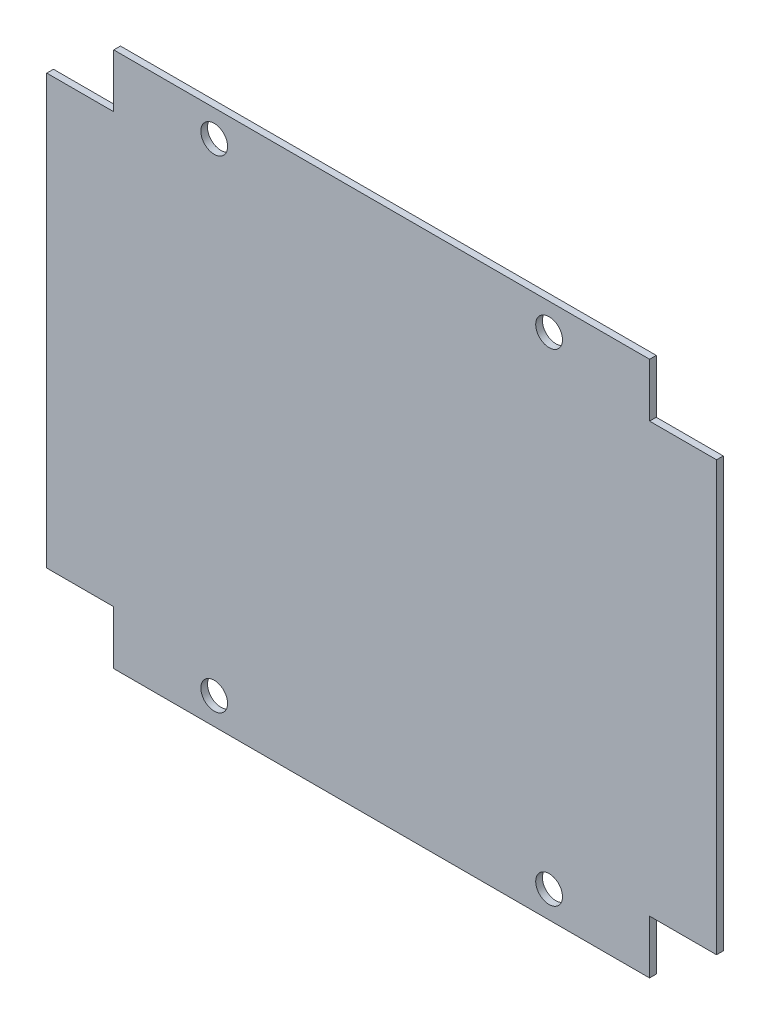
SolidWorks part; units mm, degrees
ref_plane "Front Plane" through (0, 0, 0) normal (0, 0, 1) x (1, 0, 0)
ref_plane "Top Plane" through (0, 0, 0) normal (0, 1, 0) x (1, 0, 0)
ref_plane "Right Plane" through (0, 0, 0) normal (1, 0, 0) x (0, 0, -1)
sketch "Sketch1" plane through (0, 0, 0) normal (0, 0, 1) x (1, 0, 0)
  line L0 (-40, 36) -> (40, 36) construction
  line L1 (-40, 40) -> (40, 40)
  line L2 (-50, 32) -> (-50, -32)
  line L3 (-40, -40) -> (40, -40)
  line L4 (50, 32) -> (50, -32)
  line L5 (-40, 32) -> (40, -32) construction
  line L6 (-40, -32) -> (40, 32) construction
  line L7 (0, 0) -> (35.7744, 0) construction
  line L8 (-40, -36) -> (40, -36) construction
  line L9 (-50, 32) -> (-40, 32)
  line L10 (-40, 32) -> (-40, 40)
  line L11 (-40, -32) -> (-40, -40)
  line L12 (-50, -32) -> (-40, -32)
  line L13 (0, 0) -> (0, 16.2182) construction
  line L14 (40, -32) -> (40, -40)
  line L15 (50, -32) -> (40, -32)
  line L16 (50, 32) -> (40, 32)
  line L17 (40, 32) -> (40, 40)
  circle A6 centre (-25, 36) radius 2
  circle A7 centre (-25, -36) radius 2
  circle A8 centre (25, 36) radius 2
  circle A9 centre (25, -36) radius 2
  point P0 (0, 0)
  dimension "D3" = 10
  dimension "D6" = 15
  dimension "D1" = 15
  dimension "D2" = 15
  dimension "D4" = 8
  dimension "D5" = 15
extrude "Boss-Extrude1" add sketch "Sketch1" along normal blind 1
